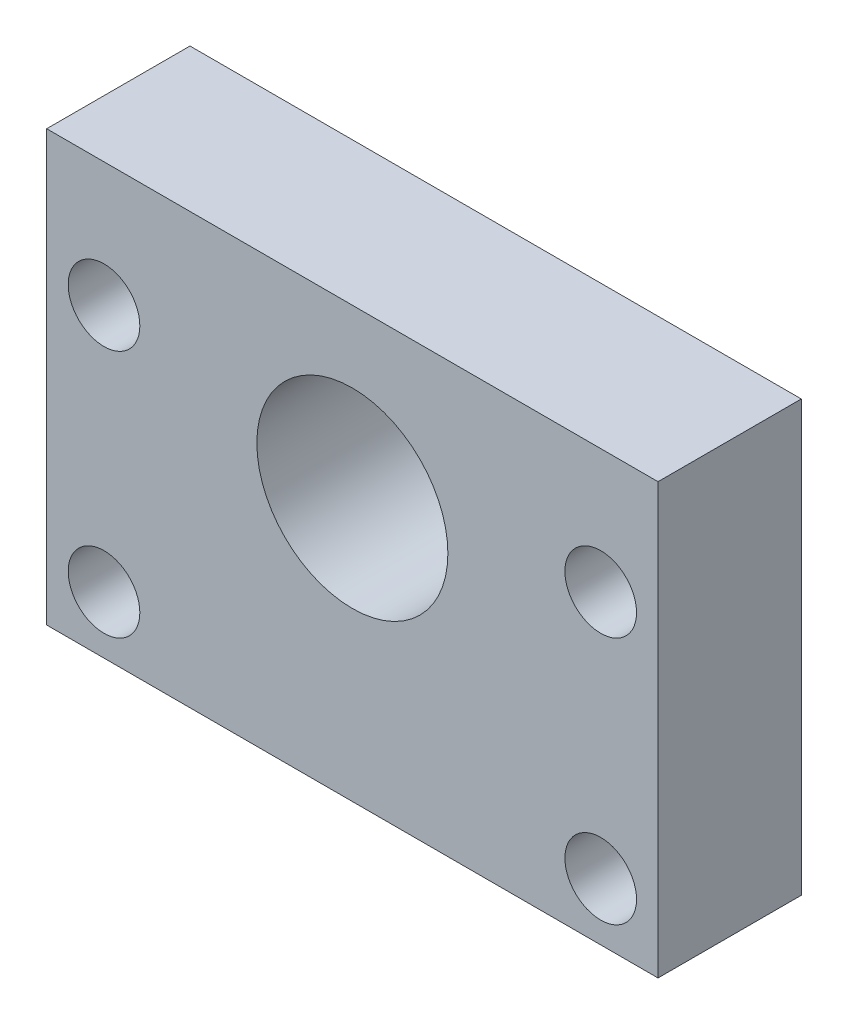
from build123d import *

# Parameters (mm, degrees)
SKETCH1_W                      = 128
SKETCH1_H                      = 90
BOSS_EXTRUDE1_DEPTH            = 30
SKETCH4_R                      = 20
CUT_EXTRUDE3_DEPTH             = 84.791407674
F_15_0_15_DIAMETER_HOLE1_D     = 15
F_15_0_15_DIAMETER_HOLE1_DEPTH = 42
F_15_0_15_DIAMETER_HOLE1_TIP   = 4.506454643


with BuildPart() as part:
    # Sketch1 → Boss-Extrude1 (new body)
    with BuildSketch(Plane.XY):
        Rectangle(SKETCH1_W, SKETCH1_H)
    extrude(amount=BOSS_EXTRUDE1_DEPTH)

    # Sketch4 → Cut-Extrude3 (cut, through all)
    with BuildSketch(Plane.XY.offset(30)):
        with Locations((0, 10)):
            Circle(SKETCH4_R)
    extrude(amount=-CUT_EXTRUDE3_DEPTH, mode=Mode.SUBTRACT)

    # Ø15.0 (15) Diameter Hole1
    with Locations(Plane.XY.offset(30)):
        with Locations((-52, 19), (-52, -33), (52, -33), (52, 19)):
            Hole(F_15_0_15_DIAMETER_HOLE1_D / 2, depth=F_15_0_15_DIAMETER_HOLE1_DEPTH)
            with Locations((0, 0, -(F_15_0_15_DIAMETER_HOLE1_DEPTH + F_15_0_15_DIAMETER_HOLE1_TIP / 2))):  # 118° drill point
                Cone(0, F_15_0_15_DIAMETER_HOLE1_D / 2, F_15_0_15_DIAMETER_HOLE1_TIP, mode=Mode.SUBTRACT)


solid = part.part
